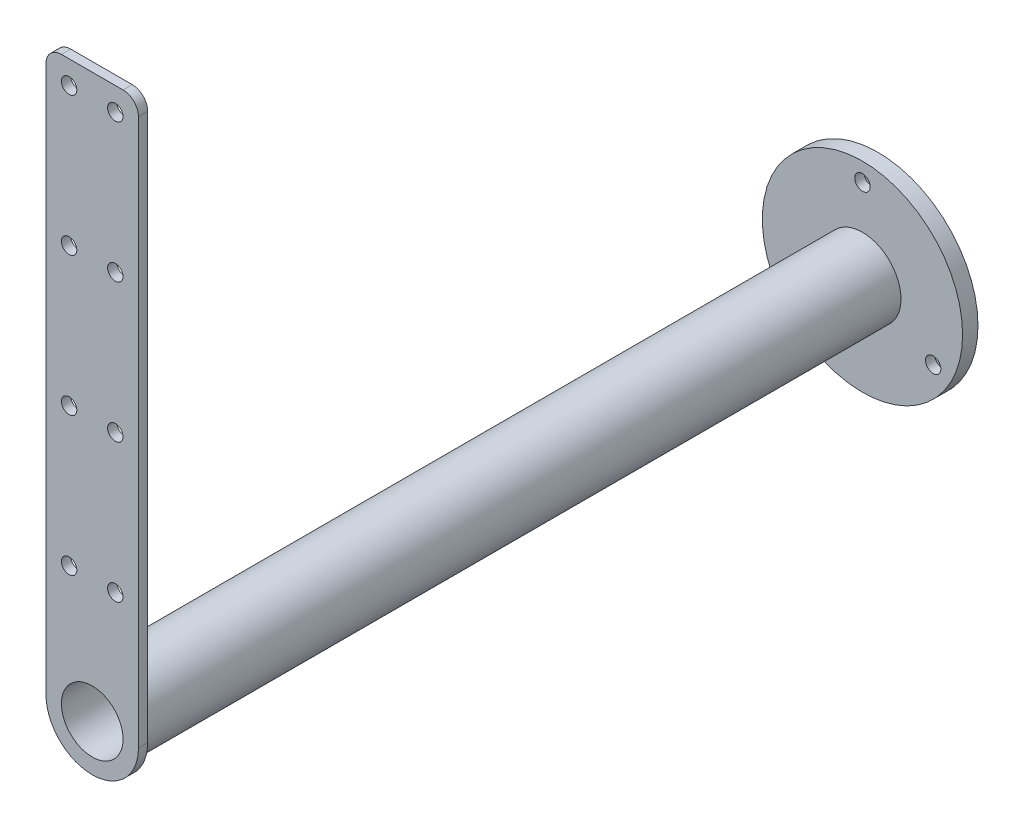
from build123d import *

# Parameters (mm, degrees)
SKETCH1_R           = 65
SKETCH1_R_2         = 20
BOSS_EXTRUDE1_DEPTH = 10
SKETCH2_R           = 25
SKETCH2_R_2         = 20
BOSS_EXTRUDE2_DEPTH = 494
SKETCH3_R           = 20
BOSS_EXTRUDE3_DEPTH = 6
FILLET1_R           = 10
SKETCH4_R           = 5
CUT_EXTRUDE1_DEPTH  = 6
SKETCH5_R           = 5
CUT_EXTRUDE2_DEPTH  = 6


with BuildPart() as part:
    # Sketch1 → Boss-Extrude1 (new body)
    with BuildSketch(Plane.XY):
        Circle(SKETCH1_R)
        Circle(SKETCH1_R_2, mode=Mode.SUBTRACT)
    extrude(amount=BOSS_EXTRUDE1_DEPTH)

    # Sketch2 → Boss-Extrude2 (add)
    with BuildSketch(Plane.XY.offset(10)):
        Circle(SKETCH2_R)
        Circle(SKETCH2_R_2, mode=Mode.SUBTRACT)
    extrude(amount=BOSS_EXTRUDE2_DEPTH)

    # Sketch3 → Boss-Extrude3 (add)
    with BuildSketch(Plane.XY.offset(504)):
        with BuildLine():
            Line((-30, 0), (-30, 365))
            Line((-30, 365), (30, 365))
            Line((30, 365), (30, 0))
            ThreePointArc((30, 0), (0, -30), (-30, 0))
        make_face()
        Circle(SKETCH3_R, mode=Mode.SUBTRACT)
    extrude(amount=BOSS_EXTRUDE3_DEPTH)

    # Fillet1
    fillet1_edges = [part.edges().sort_by_distance(p)[0] for p in [
        (30, 365, 507),
        (-30, 365, 507),
    ]]
    fillet(fillet1_edges, radius=FILLET1_R)

    # Sketch4 → Cut-Extrude1 (cut)
    with BuildSketch(Plane.XY.offset(510)):
        with Locations((-15, 350)):
            Circle(SKETCH4_R)
        with Locations((15, 350)):
            Circle(SKETCH4_R)
        with Locations((-15, 260)):
            Circle(SKETCH4_R)
        with Locations((15, 260)):
            Circle(SKETCH4_R)
        with Locations((-15, 170)):
            Circle(SKETCH4_R)
        with Locations((15, 170)):
            Circle(SKETCH4_R)
        with Locations((-15, 80)):
            Circle(SKETCH4_R)
        with Locations((15, 80)):
            Circle(SKETCH4_R)
    extrude(amount=-CUT_EXTRUDE1_DEPTH, mode=Mode.SUBTRACT)

    # Sketch5 → Cut-Extrude2 (cut)
    with BuildSketch(Plane.XY.offset(10)):
        with Locations((0, 53)):
            Circle(SKETCH5_R)
        with Locations((45.899346401, -26.5)):
            Circle(SKETCH5_R)
        with Locations((-45.899346401, -26.5)):
            Circle(SKETCH5_R)
    extrude(amount=-CUT_EXTRUDE2_DEPTH, mode=Mode.SUBTRACT)


solid = part.part
